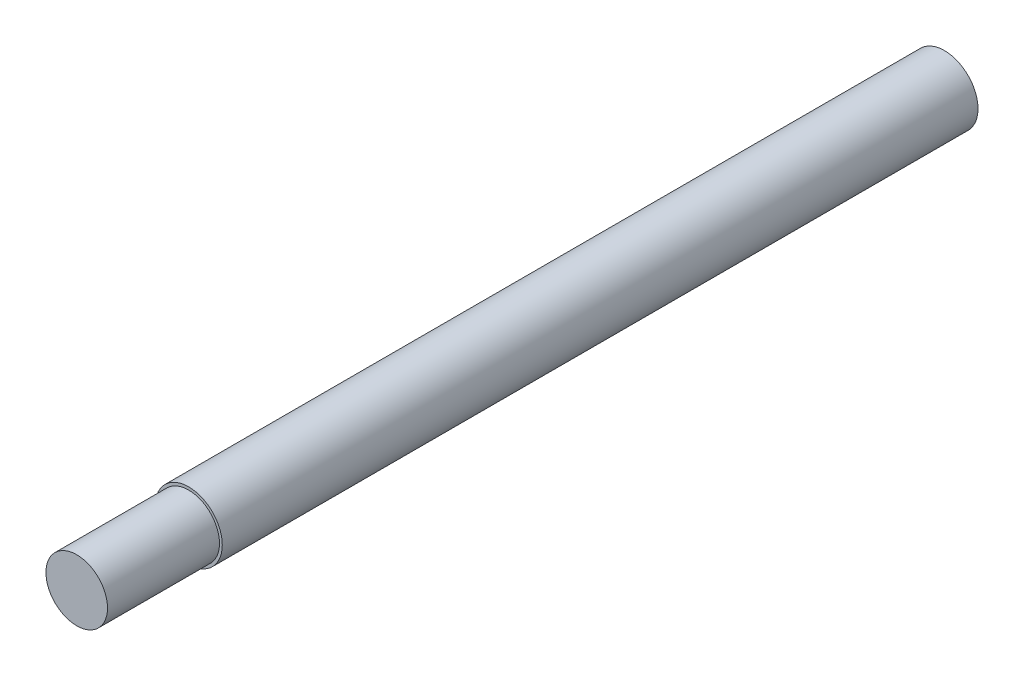
from build123d import *

# Parameters (mm, degrees)
SKETCH_1_R          = 6
EXTRUDE_3_DEPTH     = 77.5
SKETCH_3_R          = 6
SKETCH_3_R_2        = 5.5
CUT_EXTRUDE_1_DEPTH = 20


with BuildPart() as part:
    # 草图1 → 凸台-拉伸3 (new, symmetric)
    with BuildSketch(Plane.XY):
        Circle(SKETCH_1_R)
    extrude(amount=EXTRUDE_3_DEPTH, both=True)

    # 草图3 → 切除-拉伸1 (cut)
    with BuildSketch(Plane.XY.offset(77.5)):
        Circle(SKETCH_3_R)
        Circle(SKETCH_3_R_2, mode=Mode.SUBTRACT)
    extrude(amount=-CUT_EXTRUDE_1_DEPTH, mode=Mode.SUBTRACT)


solid = part.part
